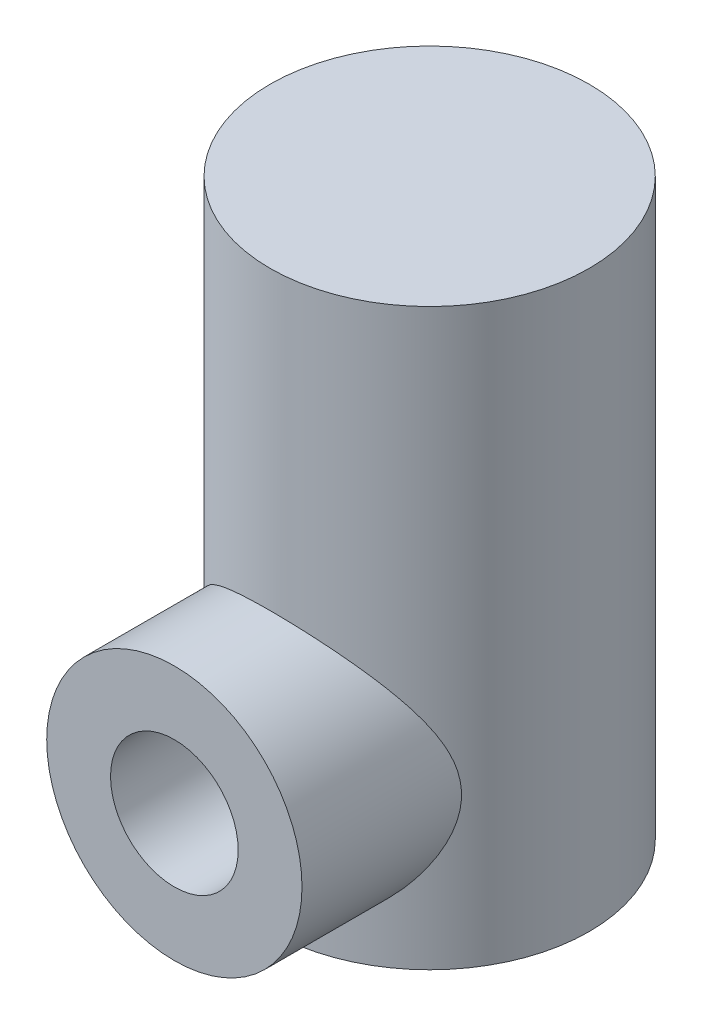
SolidWorks part; units mm, degrees
ref_plane "前视基准面" through (0, 0, 0) normal (0, 0, 1) x (1, 0, 0)
ref_plane "上视基准面" through (0, 0, 0) normal (0, 1, 0) x (1, 0, 0)
ref_plane "右视基准面" through (0, 0, 0) normal (1, 0, 0) x (0, 0, -1)
sketch "草图1" plane through (0, 0, 0) normal (0, 0, 1) x (1, 0, 0)
  circle A0 centre (2.3607, -1.2873) radius 2 construction
  circle A1 centre (2.3607, -1.2873) radius 2
  circle A2 centre (2.3607, -1.2873) radius 4
  dimension "D1" = 2
extrude "凸台-拉伸1" add sketch "草图1" along normal blind 8
sketch "草图3" plane through (0, 0, 0) normal (0, 1, 0) x (1, 0, 0)
  line L0 (6.3607, 0) -> (-1.6393, 0) construction
  circle A0 centre (2.3607, 0) radius 5
  dimension "D1" = 10
extrude "凸台-拉伸2" add sketch "草图3" along normal blind 12 and the other way blind 6
